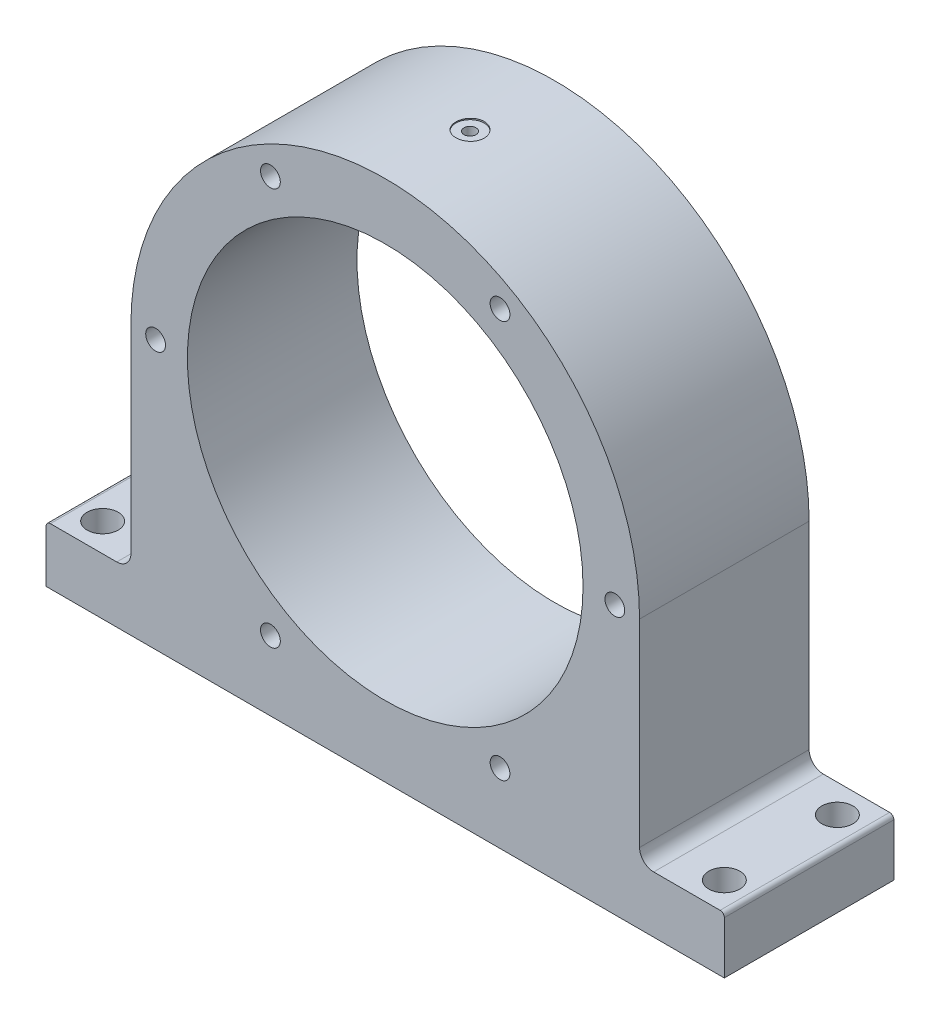
from build123d import *

# Parameters (mm, degrees)
SKETCH1_R              = 140
BOSS_EXTRUDE1_DEPTH    = 120
SKETCH3_R              = 10
CUT_EXTRUDE1_DEPTH     = 1
M10_TAPPED_HOLE1_D     = 8.5
M10_TAPPED_HOLE1_DEPTH = 40
M10_TAPPED_HOLE1_TIP   = 2.553657631
SKETCH7_R              = 11
CUT_EXTRUDE2_DEPTH     = 11303.32306496
FILLET1_R              = 3
CIRPATTERN1_COUNT      = 6
M16_TAPPED_HOLE2_D     = 14
M16_TAPPED_HOLE2_DEPTH = 38
M16_TAPPED_HOLE2_TIP   = 4.206024333


with BuildPart() as part:
    # Sketch1 → Boss-Extrude1 (new body)
    with BuildSketch(Plane.XY):
        with BuildLine():
            Line((10876.867117242, -355.960833708), (10876.867117242, -495.960833708))
            ThreePointArc((10876.867117242, -495.960833708), (10873.938185054, -503.03190152), (10866.867117242, -505.960833708))
            Line((10866.867117242, -505.960833708), (10816.867117242, -505.960833708))
            Line((10816.867117242, -505.960833708), (10816.867117242, -545.960833708))
            Line((10816.867117242, -545.960833708), (11296.867117242, -545.960833708))
            Line((11296.867117242, -545.960833708), (11296.867117242, -505.960833708))
            Line((11296.867117242, -505.960833708), (11246.867117242, -505.960833708))
            ThreePointArc((11246.867117242, -505.960833708), (11239.796049431, -503.03190152), (11236.867117242, -495.960833708))
            Line((11236.867117242, -495.960833708), (11236.867117242, -355.960833708))
            ThreePointArc((11236.867117242, -355.960833708), (11056.867117242, -175.960833708), (10876.867117242, -355.960833708))
        make_face()
        with Locations((11056.867117242, -355.960833708)):
            Circle(SKETCH1_R, mode=Mode.SUBTRACT)
    extrude(amount=BOSS_EXTRUDE1_DEPTH)

    # Sketch3 → Cut-Extrude1 (cut)
    with BuildSketch(Plane(origin=(0, -175.960833708, 0), x_dir=(1, 0, 0), z_dir=(0, 1, 0))):
        with Locations(Location((11056.867117242, -60, 0), (0, 0, 270))):
            Circle(SKETCH3_R)
    extrude(amount=-CUT_EXTRUDE1_DEPTH, mode=Mode.SUBTRACT)

    # M10 Tapped Hole1
    with Locations(Plane(origin=(0, -176.960833708, 0), x_dir=(1, 0, 0), z_dir=(0, 1, 0))):
        with Locations((11056.867117242, -60)):
            Hole(M10_TAPPED_HOLE1_D / 2, depth=M10_TAPPED_HOLE1_DEPTH)
            with Locations((0, 0, -(M10_TAPPED_HOLE1_DEPTH + M10_TAPPED_HOLE1_TIP / 2))):  # 118° drill point
                Cone(0, M10_TAPPED_HOLE1_D / 2, M10_TAPPED_HOLE1_TIP, mode=Mode.SUBTRACT)

    # Sketch7 → Cut-Extrude2 (cut, through all)
    with BuildSketch(Plane(origin=(0, -505.960833708, 0), x_dir=(1, 0, 0), z_dir=(0, 1, 0))):
        with Locations(Location((10836.867117242, -20, 0), (0, 0, 270))):
            Circle(SKETCH7_R)
        with Locations(Location((10836.867117242, -100, 0), (0, 0, 270))):
            Circle(SKETCH7_R)
        with Locations(Location((11276.867117242, -100, 0), (0, 0, 90))):
            Circle(SKETCH7_R)
        with Locations(Location((11276.867117242, -20, 0), (0, 0, 90))):
            Circle(SKETCH7_R)
    extrude(amount=-CUT_EXTRUDE2_DEPTH, mode=Mode.SUBTRACT)

    # Fillet1
    fillet1_edges = [part.edges().sort_by_distance(p)[0] for p in [
        (11296.867117242, -505.960833708, 60),
        (10816.867117242, -505.960833708, 60),
    ]]
    fillet(fillet1_edges, radius=FILLET1_R)

    # Sketch9 → M16 Tapped Hole1 (revolve, cut)
    with BuildSketch(Plane(origin=(10975.617117242, -215.231705593, 120), x_dir=(0, -1, 0), z_dir=(1, 0, 0))):
        Polygon((0, 0), (0, 42.206024333), (7, 38), (7, 0), align=None)
    m16_tapped_hole1 = revolve(axis=Axis((10975.617117242, -215.231705593, 126.35), (0, 0, -1)), mode=Mode.SUBTRACT)

    # CirPattern1: M16 Tapped Hole1 ×6 about axis
    cirpattern1_axis = Axis((11056.867117242, -355.960833708, 0), (0, 0, 1))
    for i in range(1, CIRPATTERN1_COUNT):
        add(m16_tapped_hole1.rotate(cirpattern1_axis, i * 360 / CIRPATTERN1_COUNT), mode=Mode.SUBTRACT)

    # M16 Tapped Hole2
    with Locations(Plane(origin=(0, 0, 0), x_dir=(-1, 0, 0), z_dir=(0, 0, -1))):
        with Locations((-11138.117117242, -215.231705593), (-10975.617117242, -215.231705593), (-10894.367117242, -355.960833708), (-10975.617117242, -496.689961823), (-11138.117117242, -496.689961823), (-11219.367117242, -355.960833708)):
            Hole(M16_TAPPED_HOLE2_D / 2, depth=M16_TAPPED_HOLE2_DEPTH)
            with Locations((0, 0, -(M16_TAPPED_HOLE2_DEPTH + M16_TAPPED_HOLE2_TIP / 2))):  # 118° drill point
                Cone(0, M16_TAPPED_HOLE2_D / 2, M16_TAPPED_HOLE2_TIP, mode=Mode.SUBTRACT)


solid = part.part
